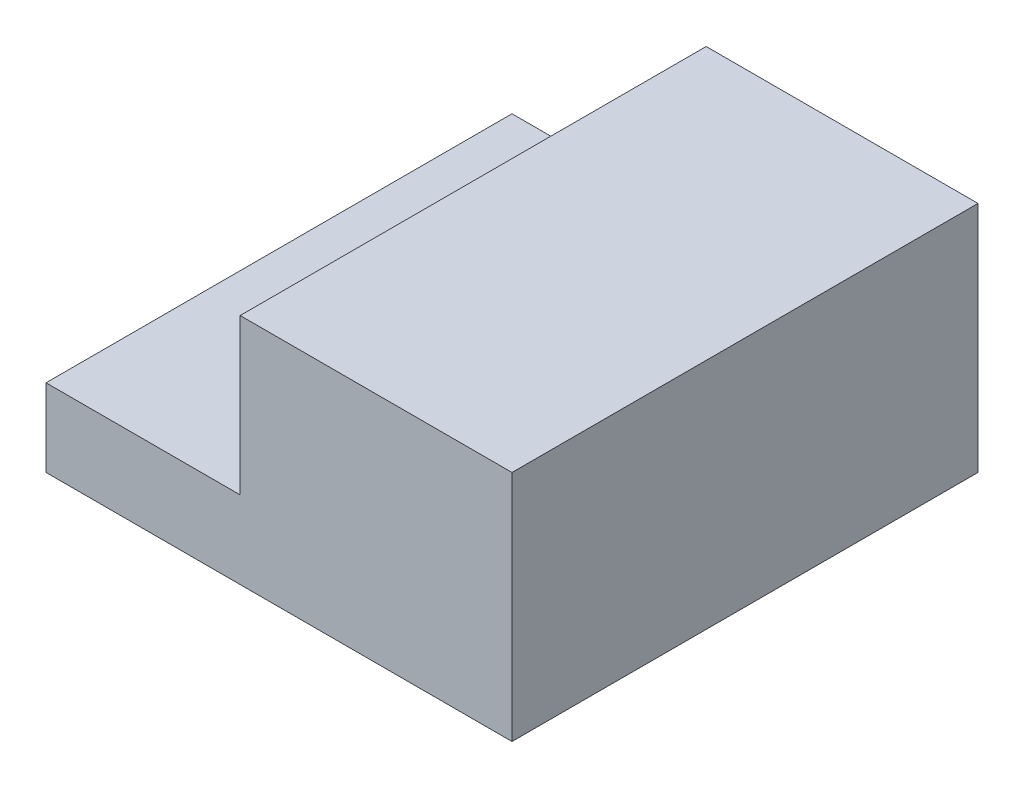
SolidWorks part; units mm, degrees
material "ABS"
ref_plane "前视基准面" through (0, 0, 0) normal (0, 0, 1) x (1, 0, 0)
ref_plane "上视基准面" through (0, 0, 0) normal (0, 1, 0) x (1, 0, 0)
ref_plane "右视基准面" through (0, 0, 0) normal (1, 0, 0) x (0, 0, -1)
other "Configuration Table"
sketch "草图1" plane through (0, 0, 0) normal (0, 0, 1) x (1, 0, 0)
  line L0 (0, 0) -> (0, 100)
  line L1 (0, 100) -> (250, 100)
  line L2 (250, 100) -> (250, 300)
  line L3 (250, 300) -> (600, 300)
  line L4 (600, 300) -> (600, 0)
  line L5 (600, 0) -> (0, 0)
  dimension "D1" = 600
  dimension "D2" = 200
  dimension "D3" = 100
  dimension "D4" = 250
extrude "凸台-拉伸1" add sketch "草图1" along normal mid plane 600
